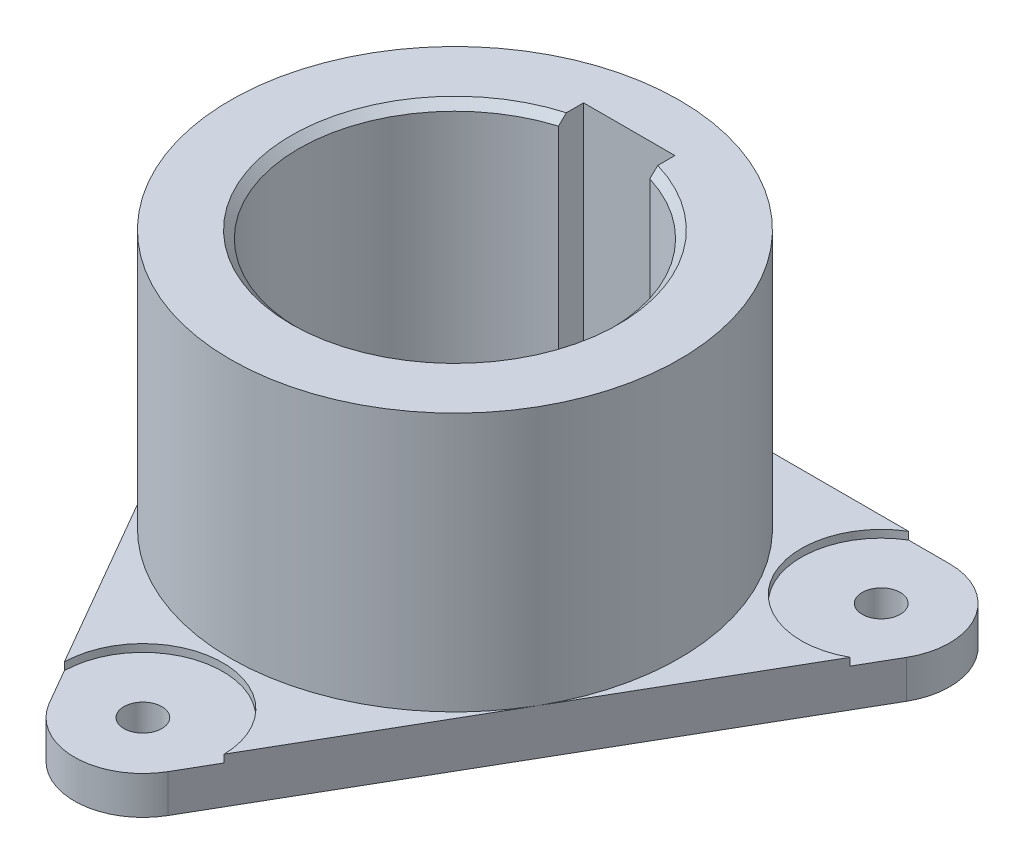
SolidWorks part; units mm, degrees
ref_plane "前视基准面" through (0, 0, 0) normal (0, 0, 1) x (1, 0, 0)
ref_plane "上视基准面" through (0, 0, 0) normal (0, 1, 0) x (1, 0, 0)
ref_plane "右视基准面" through (0, 0, 0) normal (1, 0, 0) x (0, 0, -1)
sketch "草图1" plane through (0, 0, 0) normal (0, 1, 0) x (1, 0, 0)
  line L0 (0, -13.77) -> (0, -50013.77) construction
  line L1 (22.9075, 13.2256) -> (-43278.3627, -24986.7744) construction
  line L2 (-35.507, 29.5) -> (35.507, 29.5)
  line L3 (18.0222, -10.4051) -> (43319.2924, -25010.4051) construction
  line L4 (43.3013, 16) -> (7.7942, -45.5)
  line L5 (-7.7942, -45.5) -> (-43.3013, 16)
  circle A0 centre (0, 0) radius 50 construction
  circle A1 centre (0, 0) radius 41 construction
  arc A2 (-35.507, 29.5) -> (-43.3013, 16) centre (-35.507, 20.5) ccw
  circle A3 centre (0, 0) radius 29.5
  arc A4 (43.3013, 16) -> (35.507, 29.5) centre (35.507, 20.5) ccw
  arc A5 (-7.7942, -45.5) -> (7.7942, -45.5) centre (0, -41) ccw
  dimension "D1" = 60
  dimension "D2" = 60
extrude "凸台-拉伸1" add sketch "草图1" along normal blind 6 contours A3 L2 A2 L5 | L5 A5 L4 A3 | L4 A4 L2 A3
sketch "草图2" plane through (0, 0, 0) normal (0, 1, 0) x (1, 0, 0)
  line L2 (6, 19.6023) -> (6, 22.9023)
  line L3 (6, 22.9023) -> (-6, 22.9023)
  line L4 (-6, 22.9023) -> (-6, 19.6023)
  circle A0 centre (0, 0) radius 29.5
  arc A1 (-6, 19.6023) -> (6, 19.6023) centre (0, 0) ccw
  dimension "D1" = 3.3
extrude "凸台-拉伸2" add sketch "草图2" along normal blind 40
chamfer "倒角1" distance 1 angle 45 2 edges at (0, 0, 20.5) (0, 40, 20.5)
hole_wizard "M6 螺纹孔1" positions "草图4" profile "草图3" tap size "M6" standard "Iso"
sketch "草图4" plane through (0, 6, 0) normal (0, 1, 0) x (1, 0, 0)
  point P0 (-35.507, 20.5)
  point P3 (35.507, 20.5)
  point P6 (0, -41)
sketch "草图3" plane through (-35.507, 6, -20.5) normal (1, 0, 0) x (0, 0, 1)
  line L0 (0, 0) -> (0, 16.5022)
  line L1 (0, 16.5022) -> (2.5, 15)
  line L2 (2.5, 15) -> (2.5, 0)
  line L5 (2.5, 0) -> (0, 0)
  line L10 (0, 16.5022) -> (-2.5, 15) construction
  line L11 (0, -6.35) -> (0, 107.95) construction
  dimension "螺纹孔钻头直径" = 5
  dimension "螺纹孔钻头深度" = 15
  dimension "导头角度" = 118
cosmetic thread "孔螺蚊线1" parameters "D1"=5, "D2"=6
cosmetic thread "孔螺蚊线2" parameters "D1"=5, "D2"=6
cosmetic thread "孔螺蚊线3" parameters "D1"=5, "D2"=6
sketch "草图5" plane through (0, 6, 0) normal (0, 1, 0) x (1, 0, 0)
  circle A0 centre (-35.507, 20.5) radius 10.5
  circle A1 centre (35.507, 20.5) radius 10.5
  circle A2 centre (0, -41) radius 10.5
extrude "切除-拉伸1" cut sketch "草图5" against normal blind 1
